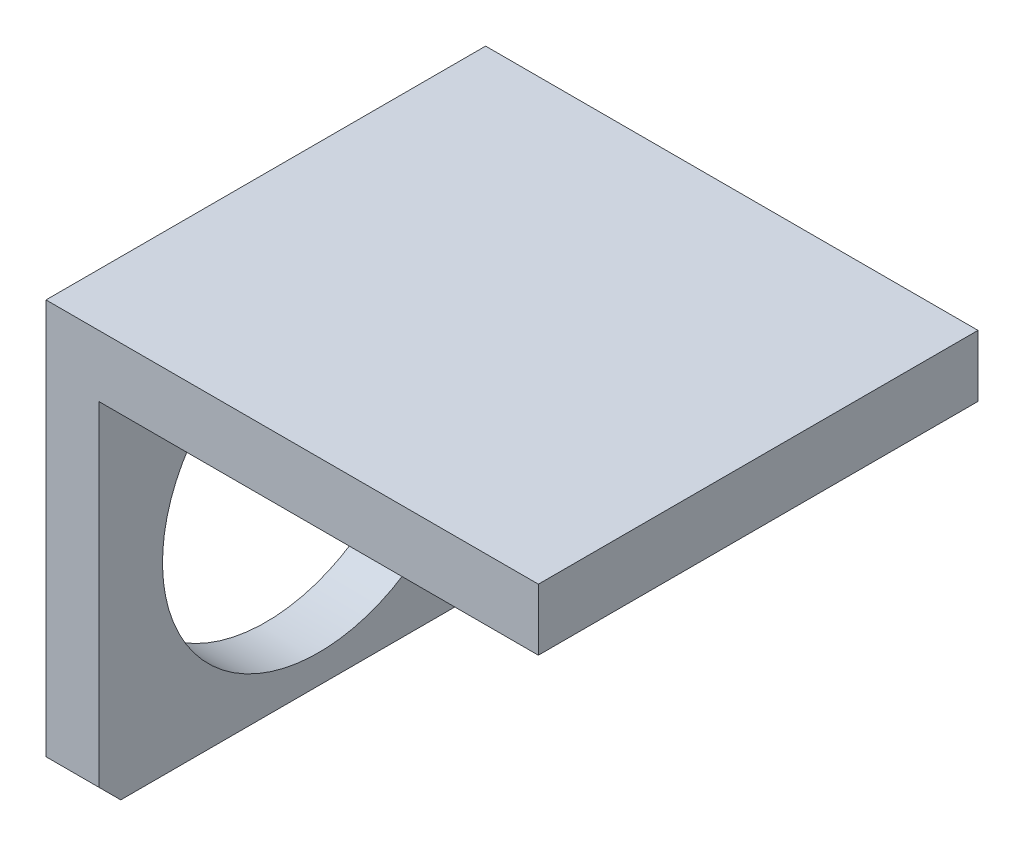
from build123d import *

# Parameters (mm, degrees)
SKETCH_1_W          = 12
SKETCH_1_H          = 95
EXTRUDE_1_DEPTH     = 50
CUT_EXTRUDE_1_REACH = 110.023
SKETCH_2_R          = 35.5
SKETCH_3_W          = 100
SKETCH_3_H          = 14
EXTRUDE_2_DEPTH     = 100
CHAMFER_1_SIZE      = 5


with BuildPart() as part:
    # 草图1 → 凸台-拉伸1 (new, symmetric)
    with BuildSketch(Plane.XY):
        with Locations((6, 47.5)):
            Rectangle(SKETCH_1_W, SKETCH_1_H)
    extrude(amount=EXTRUDE_1_DEPTH, both=True)

    # 草图2 → 切除-拉伸1 (cut, up to next)
    with BuildSketch(Plane(origin=(12, 0, 0), x_dir=(0, 0, -1), z_dir=(1, 0, 0)), mode=Mode.PRIVATE) as cut_extrude_1_sk1:
        with Locations(Location((0, 42, 0), (0, 0, 90))):
            Circle(SKETCH_2_R)
    cut_extrude_1_tool1 = extrude(cut_extrude_1_sk1.sketch, amount=-CUT_EXTRUDE_1_REACH, mode=Mode.PRIVATE) & part.part
    add(cut_extrude_1_tool1.solids().sort_by_distance((12, 42, 0))[0], mode=Mode.SUBTRACT)

    # 草图3 → 凸台-拉伸2 (add)
    with BuildSketch(Plane(origin=(12, 0, 0), x_dir=(0, 0, -1), z_dir=(1, 0, 0))):
        with Locations((0, 88)):
            Rectangle(SKETCH_3_W, SKETCH_3_H)
    extrude(amount=EXTRUDE_2_DEPTH)

    # 倒角1
    chamfer_1_edges = [part.edges().sort_by_distance(p)[0] for p in [
        (6, 0, 50),
        (6, 0, -50),
    ]]
    chamfer(chamfer_1_edges, length=CHAMFER_1_SIZE)


solid = part.part
